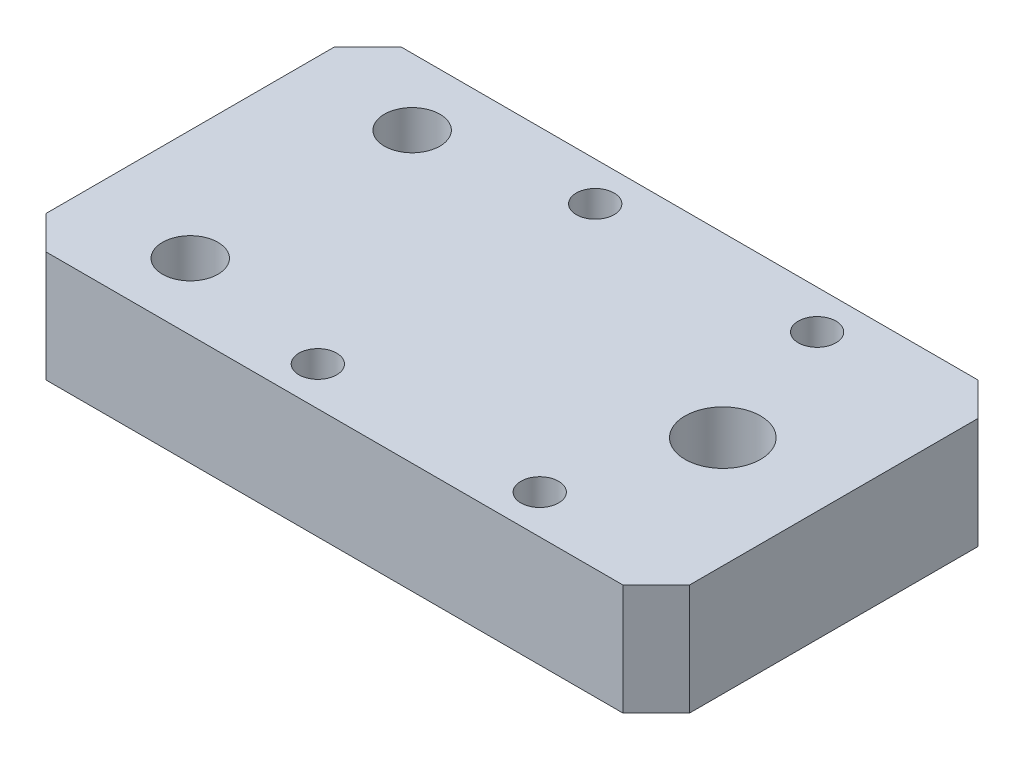
SolidWorks part; units mm, degrees
ref_plane "Front Plane" through (0, 0, 0) normal (0, 0, 1) x (1, 0, 0)
ref_plane "Top Plane" through (0, 0, 0) normal (0, 1, 0) x (1, 0, 0)
ref_plane "Right Plane" through (0, 0, 0) normal (1, 0, 0) x (0, 0, -1)
other "Configuration Table"
sketch "Sketch1" plane through (0, 0, 0) normal (0, 1, 0) x (1, 0, 0)
  line L1 (-29, 16) -> (29, 16)
  line L2 (-29, 16) -> (-29, -16)
  line L3 (-29, -16) -> (29, -16)
  line L4 (29, 16) -> (29, -16)
  line L5 (-29, 16) -> (29, -16) construction
  line L6 (-29, -16) -> (29, 16) construction
  point P0 (0, 0)
  dimension "D1" = 32
  dimension "D2" = 58
extrude "Boss-Extrude1" add sketch "Sketch1" along normal blind 10
hole_wizard "CBORE for M4 Hexagon socket head cap screws1" positions "Sketch4" profile "Sketch5" counterbore size "M3" standard "GB"
sketch "Sketch4" plane through (0, 0, 0) normal (0, -1, 0) x (-1, 0, 0)
  line L0 (29, -16) -> (-29, -16) construction
  line L1 (-29, -16) -> (-29, 16) construction
  point P0 (-15, 12.5)
  point P3 (5, 12.5)
  point P6 (-15, -12.5)
  point P9 (5, -12.5)
  dimension "D1" = 25
  dimension "D2" = 20
  dimension "D3" = 3.5
  dimension "D4" = 14
sketch "Sketch5" plane through (15, 0, -12.5) normal (1, 0, 0) x (0, 0, -1)
  line L0 (0, 0) -> (0, 19.1215)
  line L1 (0, 19.1215) -> (1.7, 18.1)
  line L2 (1.7, 18.1) -> (1.7, 3.4)
  line L3 (1.7, 3.4) -> (3, 3.4)
  line L4 (3, 3.4) -> (3, 0)
  line L5 (3, 0) -> (0, 0)
  line L10 (0, 19.1215) -> (-1.7, 18.1) construction
  line L11 (0, -6.35) -> (0, 107.95) construction
  dimension "孔直径" = 3.4
  dimension "孔深度" = 18.1
  dimension "柱形沉头孔直径" = 6
  dimension "柱形沉头孔深度" = 3.4
  dimension "导头角度" = 118
hole_wizard "M6 Tapped Hole1" positions "Sketch7" profile "Sketch8" tap size "M6" standard "GB"
sketch "Sketch7" plane through (0, 0, 0) normal (0, -1, 0) x (-1, 0, 0)
  line L0 (29, 16) -> (29, -16) construction
  point P0 (19, 10)
  point P2 (19, -10)
  dimension "D1" = 20
  dimension "D2" = 10
  dimension "D3" = 10
sketch "Sketch8" plane through (-19, 0, -10) normal (1, 0, 0) x (0, 0, -1)
  line L0 (0, 0) -> (0, 16.5022)
  line L1 (0, 16.5022) -> (2.5, 15)
  line L2 (2.5, 15) -> (2.5, 0)
  line L5 (2.5, 0) -> (0, 0)
  line L10 (0, 16.5022) -> (-2.5, 15) construction
  line L11 (0, -6.35) -> (0, 107.95) construction
  dimension "螺纹孔钻头直径" = 5
  dimension "螺纹孔钻头深度" = 15
  dimension "导头角度" = 118
cosmetic thread "Cosmetic Thread1"
cosmetic thread "Cosmetic Thread2"
hole_wizard "M8 Tapped Hole1" positions "Sketch9" profile "Sketch10" tap size "M8" standard "GB"
sketch "Sketch9" plane through (0, 0, 0) normal (0, -1, 0) x (-1, 0, 0)
  line L0 (-29, -16) -> (-29, 16) construction
  point P0 (-19, 0)
  dimension "D1" = 10
sketch "Sketch10" plane through (19, 0, 0) normal (1, 0, 0) x (0, 0, -1)
  line L0 (0, 0) -> (0, 21.7929)
  line L1 (0, 21.7929) -> (3.4, 19.75)
  line L2 (3.4, 19.75) -> (3.4, 0)
  line L5 (3.4, 0) -> (0, 0)
  line L10 (0, 21.7929) -> (-3.4, 19.75) construction
  line L11 (0, -6.35) -> (0, 107.95) construction
  dimension "螺纹孔钻头直径" = 6.8
  dimension "螺纹孔钻头深度" = 19.75
  dimension "导头角度" = 118
cosmetic thread "Cosmetic Thread3" parameters "D1"=16, "D2"=8
chamfer "Chamfer1" distance 3 angle 45 4 edges at (-29, 5, -16) (29, 5, -16) (-29, 5, 16) (29, 5, 16)
